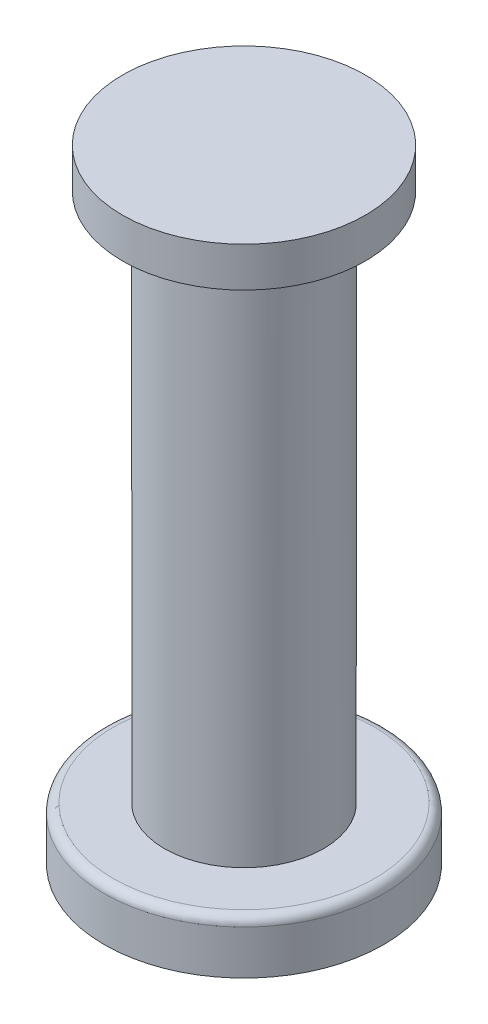
SolidWorks part; units mm, degrees
ref_plane "Front Plane" through (0, 0, 0) normal (0, 0, 1) x (1, 0, 0)
ref_plane "Top Plane" through (0, 0, 0) normal (0, 1, 0) x (1, 0, 0)
ref_plane "Right Plane" through (0, 0, 0) normal (1, 0, 0) x (0, 0, -1)
sketch "Sketch1" plane through (0, 0, 0) normal (0, 1, 0) x (1, 0, 0)
  circle A0 centre (0, 0) radius 137.5
  dimension "D1" = 275
extrude "Boss-Extrude1" add sketch "Sketch1" along normal blind 45
sketch "Sketch2" plane through (0, 0, 0) normal (0, -1, 0) x (1, 0, 0)
  circle A0 centre (0, 0) radius 90
  dimension "D1" = 180
extrude "Boss-Extrude2" add sketch "Sketch2" along normal blind 600
sketch "Sketch3" plane through (0, -600, 0) normal (0, -1, 0) x (1, 0, 0)
  circle A0 centre (0, 0) radius 158.1822
extrude "Boss-Extrude3" add sketch "Sketch3" along normal blind 60
fillet "Fillet1" radius 10 1 edges at (0, -600, -158.1822)
